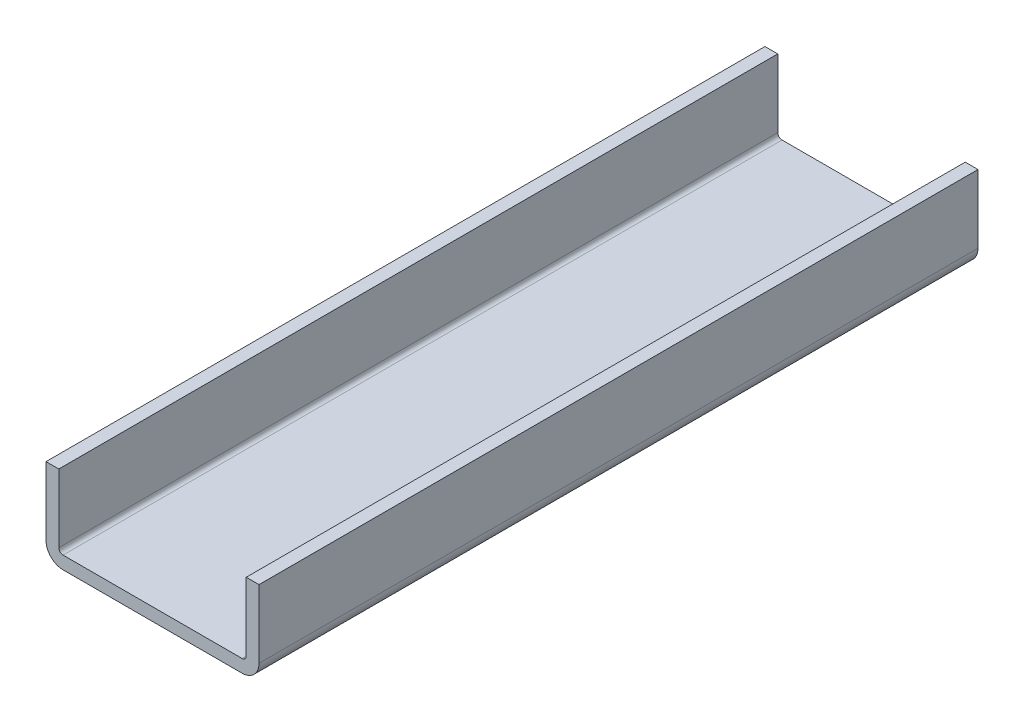
SolidWorks part; units mm, degrees
material "1023 Carbon Steel Plate (SS)"
ref_plane "Front Plane" through (0, 0, 0) normal (0, 0, 1) x (1, 0, 0)
ref_plane "Top Plane" through (0, 0, 0) normal (0, 1, 0) x (1, 0, 0)
ref_plane "Right Plane" through (0, 0, 0) normal (1, 0, 0) x (0, 0, -1)
sketch "Sketch2" plane through (0, 0, 0) normal (0, 0, 1) x (1, 0, 0)
  line L0 (0, 0) -> (0, -32)
  line L1 (8, -40) -> (92, -40)
  line L2 (100, -32) -> (100, 0)
  line L3 (6, 0) -> (6, -32)
  line L4 (8, -34) -> (92, -34)
  line L5 (94, -32) -> (94, 0)
  line L6 (6, 0) -> (0, 0)
  line L7 (100, 0) -> (94, 0)
  arc A0 (92, -40) -> (100, -32) centre (92, -32) ccw
  arc A1 (0, -32) -> (8, -40) centre (8, -32) ccw
  arc A2 (6, -32) -> (8, -34) centre (8, -32) ccw
  arc A3 (92, -34) -> (94, -32) centre (92, -32) ccw
  point P7 (100, -40)
  point P10 (0, -40)
  dimension "D4" = 8
  dimension "D1" = 40
  dimension "D2" = 100
  dimension "D3" = 40
  dimension "D5" = 6
extrude "Boss-Extrude2" add sketch "Sketch2" along normal blind 337.5 contours L7 L5 A3 L4 A2 L3 L6 L0 A1 L1 A0 L2
